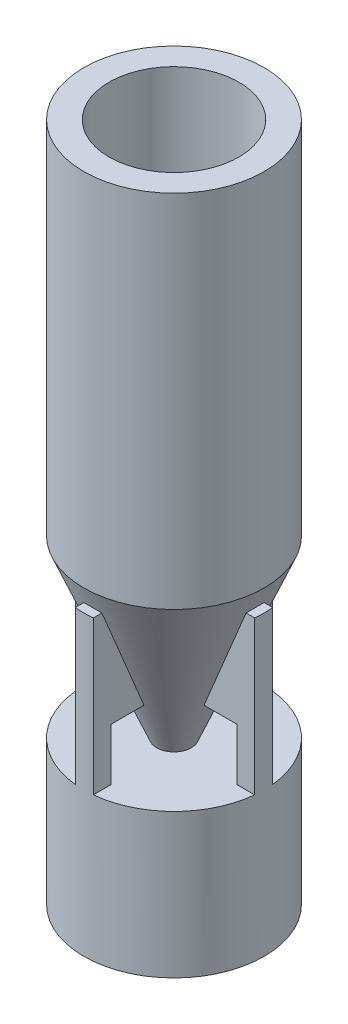
SolidWorks part; units mm, degrees
ref_plane "Front Plane" through (0, 0, 0) normal (0, 0, 1) x (1, 0, 0)
ref_plane "Top Plane" through (0, 0, 0) normal (0, 1, 0) x (1, 0, 0)
ref_plane "Right Plane" through (0, 0, 0) normal (1, 0, 0) x (0, 0, -1)
sketch "Sketch1" plane through (0, 0, 0) normal (0, 0, 1) x (1, 0, 0)
  line L0 (0, 0) -> (0, 1600)
  line L1 (0, 1600) -> (250, 1600)
  line L2 (250, 1600) -> (250, 600)
  line L3 (250, 600) -> (0, 0)
  dimension "D1" = 250
  dimension "D2" = 1600
  dimension "D3" = 1000
revolve "Revolve1" add sketch "Sketch1" angle 360 about L0
shell "Shell1" thickness 70
sketch "Sketch2" plane through (0, 0, 0) normal (0, 0, 1) x (1, 0, 0)
  line L0 (0, 0) -> (0, 540) construction
  line L1 (0, 540) -> (-338.6452, 540) construction
  line L3 (-250, 600) -> (0, 0) construction
  line L4 (-108.3333, 260) -> (-199.3333, 260)
  line L5 (-199.3333, 260) -> (-199.3333, 0)
  line L6 (-199.3333, 0) -> (-250, 0)
  line L7 (-225, 540) -> (-108.3333, 260)
  line L8 (225, 540) -> (108.3333, 260)
  line L9 (199.3333, 0) -> (250, 0)
  line L10 (199.3333, 260) -> (199.3333, 0)
  line L11 (108.3333, 260) -> (199.3333, 260)
  line L13 (-225, 540) -> (-250, 540)
  line L14 (-250, 540) -> (-250, 0)
  line L15 (225, 540) -> (250, 540)
  line L16 (250, 540) -> (250, 0)
  dimension "D1" = 540
  dimension "D2" = 250
  dimension "D3" = 91
  dimension "D4" = 260
extrude "Boss-Extrude1" add sketch "Sketch2" along normal mid plane 50 separate body
sketch "Sketch3" plane through (0, 0, 0) normal (1, 0, 0) x (0, 0, -1)
  line L1 (-250, 600) -> (0, 0) construction
  line L2 (-250, 0) -> (-199.3333, 0)
  line L3 (-199.3333, 0) -> (-199.3333, 260)
  line L4 (-199.3333, 260) -> (-108.3333, 260)
  line L5 (-108.3333, 260) -> (-225, 540)
  line L6 (0, 0) -> (0, 692.8002) construction
  line L7 (108.3333, 260) -> (225, 540)
  line L8 (199.3333, 260) -> (108.3333, 260)
  line L9 (199.3333, 0) -> (199.3333, 260)
  line L10 (250, 0) -> (199.3333, 0)
  line L12 (-225, 540) -> (-250, 540)
  line L13 (-250, 540) -> (-250, 0)
  line L14 (250, 540) -> (250, 0)
  line L15 (225, 540) -> (250, 540)
  dimension "D1" = 260
  dimension "D2" = 250
  dimension "D3" = 91
  dimension "D4" = 540
extrude "Boss-Extrude2" add sketch "Sketch3" along normal mid plane 50 separate body
sketch "Sketch4" plane through (0, 0, 0) normal (0, 0, 1) x (1, 0, 0)
  line L0 (250, 115) -> (0, 115)
  line L1 (0, 115) -> (0, -285)
  line L2 (0, -285) -> (250, -285)
  line L3 (250, -285) -> (250, 115)
  line L4 (108.3333, 260) -> (199.3333, 260) construction
  dimension "D1" = 400
  dimension "D2" = 145
  dimension "D3" = 250
revolve "Revolve2" add sketch "Sketch4" angle 360 about L1
sketch "Sketch5" plane through (0, -285, 0) normal (0, -1, 0) x (1, 0, 0)
  circle A1 centre (0, 0) radius 250
  circle A2 centre (0, 0) radius 250
  dimension "D1" = 0
extrude "Cut-Extrude1" cut sketch "Sketch5" against normal through all flip side to cut
